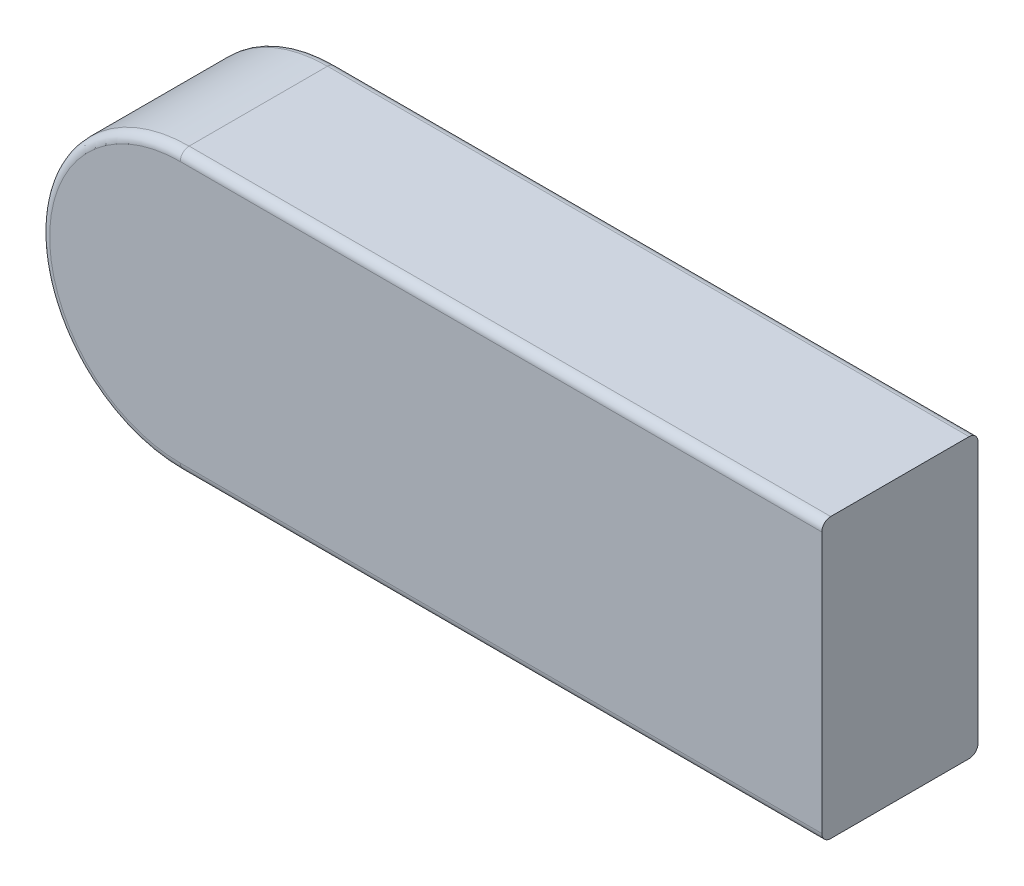
from build123d import *

# Parameters (mm, degrees)
EXTRUDE_494_DEPTH = 14
FILLET_1_R        = 0.8


with BuildPart() as part:
    # 草图1 → Extrude 494 (new body)
    with BuildSketch(Plane.XY):
        with BuildLine():
            Line((-9, 12.5), (48.5, 12.5))
            Line((48.5, 12.5), (48.5, -12.5))
            Line((48.5, -12.5), (-9, -12.5))
            ThreePointArc((-9, -12.5), (-21.5, 0), (-9, 12.5))
        make_face()
    extrude(amount=EXTRUDE_494_DEPTH)

    # 圆角1
    fillet_1_edges = [part.edges().sort_by_distance(p)[0] for p in [
        (-21.5, 0, 14),
        (19.75, -12.5, 14),
        (19.75, -12.5, 0),
        (-21.5, 0, 0),
        (19.75, 12.5, 0),
        (19.75, 12.5, 14),
    ]]
    fillet(fillet_1_edges, radius=FILLET_1_R)


solid = part.part
